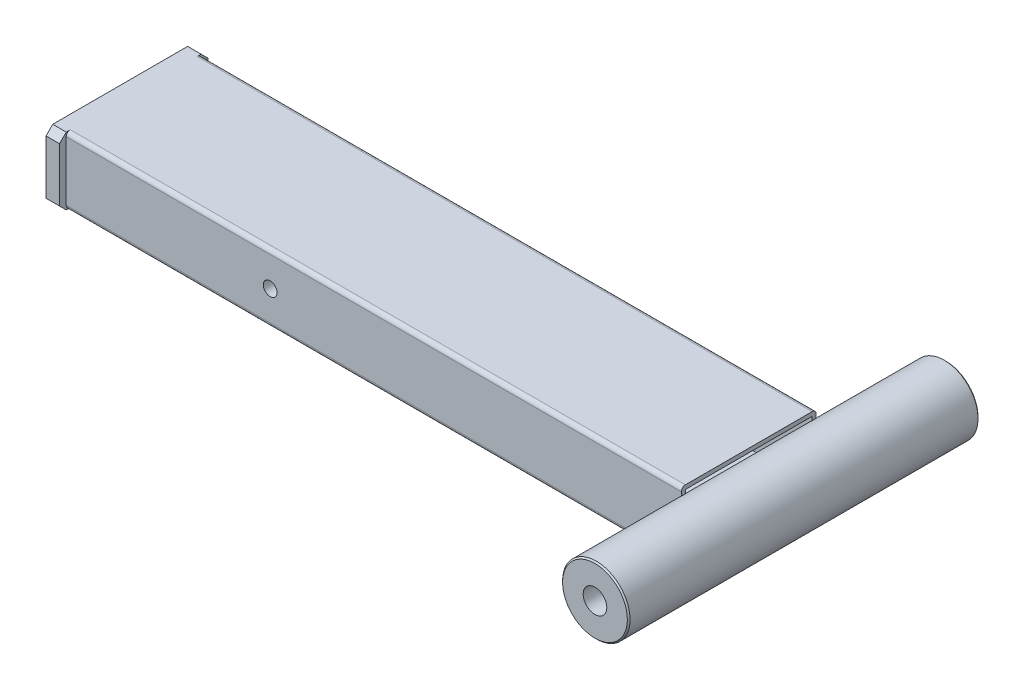
from build123d import *

# Parameters (mm, degrees)
SKETCH_1_W                    = 466
SKETCH_1_H                    = 110
EXTRUDE_1_DEPTH               = 50
SKETCH_2_W                    = 456
SKETCH_2_H                    = 5
CUT_EXTRUDE_1_DEPTH           = 250.337121183
SKETCH_3_W                    = 456
SKETCH_3_H                    = 5
CUT_EXTRUDE_2_DEPTH           = 250.337121183
SKETCH_4_W                    = 94
SKETCH_4_H                    = 44
CUT_EXTRUDE_3_DEPTH           = 456
SKETCH_5_W                    = 10
SKETCH_5_H                    = 94
SKETCH_6_W                    = 25
SKETCH_6_H                    = 260
HOLE_WIZARD_8_5_8_5_1_D       = 8.5
HOLE_WIZARD_8_5_8_5_1_DEPTH   = 10
HOLE_WIZARD_M12_3_D           = 10.2
HOLE_WIZARD_M12_3_DEPTH       = 29.25
HOLE_WIZARD_M12_3_TIP         = 3.064389157
HOLE_WIZARD_M12_4_D           = 10.2
HOLE_WIZARD_M12_4_DEPTH       = 29.25
HOLE_WIZARD_M12_4_TIP         = 3.064389157
HOLE_WIZARD_10_2_10_2_2_D     = 10.2
HOLE_WIZARD_10_2_10_2_2_DEPTH = 29.25
HOLE_WIZARD_10_2_10_2_2_TIP   = 3.064389157
CHAMFER_1_SIZE                = 1
FILLET_1_R                    = 3
CHAMFER_2_SIZE                = 5
HOLE_WIZARD_M20_1_D           = 17.5
HOLE_WIZARD_M20_1_DEPTH       = 47.5
HOLE_WIZARD_M20_1_TIP         = 5.257530416
HOLE_WIZARD_M20_2_D           = 17.5
HOLE_WIZARD_M20_2_DEPTH       = 47.5
HOLE_WIZARD_M20_2_TIP         = 5.257530416


with BuildPart() as part:
    # 草图1 → 凸台-拉伸1 (new body)
    with BuildSketch(Plane(origin=(0, 25, 0), x_dir=(1, 0, 0), z_dir=(0, 1, 0))):
        with Locations((-5, 0)):
            Rectangle(SKETCH_1_W, SKETCH_1_H)
    extrude(amount=-EXTRUDE_1_DEPTH)

    # 草图2 → 切除-拉伸1 (cut, through all)
    with BuildSketch(Plane.XZ.offset(25)):
        with Locations((0, -52.5)):
            Rectangle(SKETCH_2_W, SKETCH_2_H)
    extrude(amount=-CUT_EXTRUDE_1_DEPTH, mode=Mode.SUBTRACT)

    # 草图3 → 切除-拉伸2 (cut, through all)
    with BuildSketch(Plane.XZ.offset(25)):
        with Locations((0, 52.5)):
            Rectangle(SKETCH_3_W, SKETCH_3_H)
    extrude(amount=-CUT_EXTRUDE_2_DEPTH, mode=Mode.SUBTRACT)

    # 草图4 → 切除-拉伸3 (cut)
    with BuildSketch(Plane(origin=(228, 0, 0), x_dir=(0, 0, -1), z_dir=(1, 0, 0))):
        Rectangle(SKETCH_4_W, SKETCH_4_H)
    extrude(amount=-CUT_EXTRUDE_3_DEPTH, mode=Mode.SUBTRACT)

    # 草图5 → 旋转1 (revolve)
    with BuildSketch(Plane.XZ, mode=Mode.PRIVATE) as revolve_1_sk:
        with Locations((-71.8, 0)):
            Rectangle(SKETCH_5_W, SKETCH_5_H)
    revolve(revolve_1_sk.sketch.rotate(Axis((-76.8, 0, 47), (0, 0, -1)), 180), axis=Axis((-76.8, 0, 47), (0, 0, -1)))

    # 草图6 → 旋转2 (revolve)
    with BuildSketch(Plane(origin=(0, 0, 0), x_dir=(1, 0, 0), z_dir=(0, 1, 0))):
        with Locations((231.5, 0)):
            Rectangle(SKETCH_6_W, SKETCH_6_H)
    revolve(axis=Axis((244, 0, 130), (0, 0, -1)))

    # Ø8.5 (8.5) 直径孔1
    with Locations(Plane(origin=(-228, 0, 0), x_dir=(0, 0, -1), z_dir=(1, 0, 0))):
        with Locations((40, 10), (-40, 10)):
            Hole(HOLE_WIZARD_8_5_8_5_1_D / 2, depth=HOLE_WIZARD_8_5_8_5_1_DEPTH)

    # M12 螺纹孔3
    with Locations(Plane.XY.offset(50)):
        with Locations((-76.8, 0)):
            Hole(HOLE_WIZARD_M12_3_D / 2, depth=HOLE_WIZARD_M12_3_DEPTH)
            with Locations((0, 0, -(HOLE_WIZARD_M12_3_DEPTH + HOLE_WIZARD_M12_3_TIP / 2))):  # 118° drill point
                Cone(0, HOLE_WIZARD_M12_3_D / 2, HOLE_WIZARD_M12_3_TIP, mode=Mode.SUBTRACT)

    # M12 螺纹孔4
    with Locations(Plane(origin=(0, 0, -50), x_dir=(-1, 0, 0), z_dir=(0, 0, -1))):
        with Locations((76.8, 0)):
            Hole(HOLE_WIZARD_M12_4_D / 2, depth=HOLE_WIZARD_M12_4_DEPTH)
            with Locations((0, 0, -(HOLE_WIZARD_M12_4_DEPTH + HOLE_WIZARD_M12_4_TIP / 2))):  # 118° drill point
                Cone(0, HOLE_WIZARD_M12_4_D / 2, HOLE_WIZARD_M12_4_TIP, mode=Mode.SUBTRACT)

    # Ø10.2 (10.2) 直径孔2
    with Locations(Plane(origin=(0, 0, -50), x_dir=(-1, 0, 0), z_dir=(0, 0, -1))):
        with Locations((76.8, 0)):
            Hole(HOLE_WIZARD_10_2_10_2_2_D / 2, depth=HOLE_WIZARD_10_2_10_2_2_DEPTH)
            with Locations((0, 0, -(HOLE_WIZARD_10_2_10_2_2_DEPTH + HOLE_WIZARD_10_2_10_2_2_TIP / 2))):  # 118° drill point
                Cone(0, HOLE_WIZARD_10_2_10_2_2_D / 2, HOLE_WIZARD_10_2_10_2_2_TIP, mode=Mode.SUBTRACT)

    # 倒角1
    chamfer_1_edges = [part.edges().sort_by_distance(p)[0] for p in [
        (269, 0, 130),
        (269, 0, -130),
    ]]
    chamfer(chamfer_1_edges, length=CHAMFER_1_SIZE)

    # 圆角1
    fillet_1_edges = [part.edges().sort_by_distance(p)[0] for p in [
        (0, 25, -50),
        (0, -25, -50),
        (0, 25, 50),
        (0, -25, 50),
    ]]
    fillet(fillet_1_edges, radius=FILLET_1_R)

    # 倒角2
    chamfer_2_edges = [part.edges().sort_by_distance(p)[0] for p in [
        (-233, 25, -55),
        (-233, -25, -55),
        (-233, -25, 55),
        (-233, 25, 55),
    ]]
    chamfer(chamfer_2_edges, length=CHAMFER_2_SIZE)

    # M20 螺纹孔1
    with Locations(Plane.XY.offset(130)):
        with Locations((244, 0)):
            Hole(HOLE_WIZARD_M20_1_D / 2, depth=HOLE_WIZARD_M20_1_DEPTH)
            with Locations((0, 0, -(HOLE_WIZARD_M20_1_DEPTH + HOLE_WIZARD_M20_1_TIP / 2))):  # 118° drill point
                Cone(0, HOLE_WIZARD_M20_1_D / 2, HOLE_WIZARD_M20_1_TIP, mode=Mode.SUBTRACT)

    # M20 螺纹孔2
    with Locations(Plane(origin=(0, 0, -130), x_dir=(-1, 0, 0), z_dir=(0, 0, -1))):
        with Locations((-244, 0)):
            Hole(HOLE_WIZARD_M20_2_D / 2, depth=HOLE_WIZARD_M20_2_DEPTH)
            with Locations((0, 0, -(HOLE_WIZARD_M20_2_DEPTH + HOLE_WIZARD_M20_2_TIP / 2))):  # 118° drill point
                Cone(0, HOLE_WIZARD_M20_2_D / 2, HOLE_WIZARD_M20_2_TIP, mode=Mode.SUBTRACT)


solid = part.part
